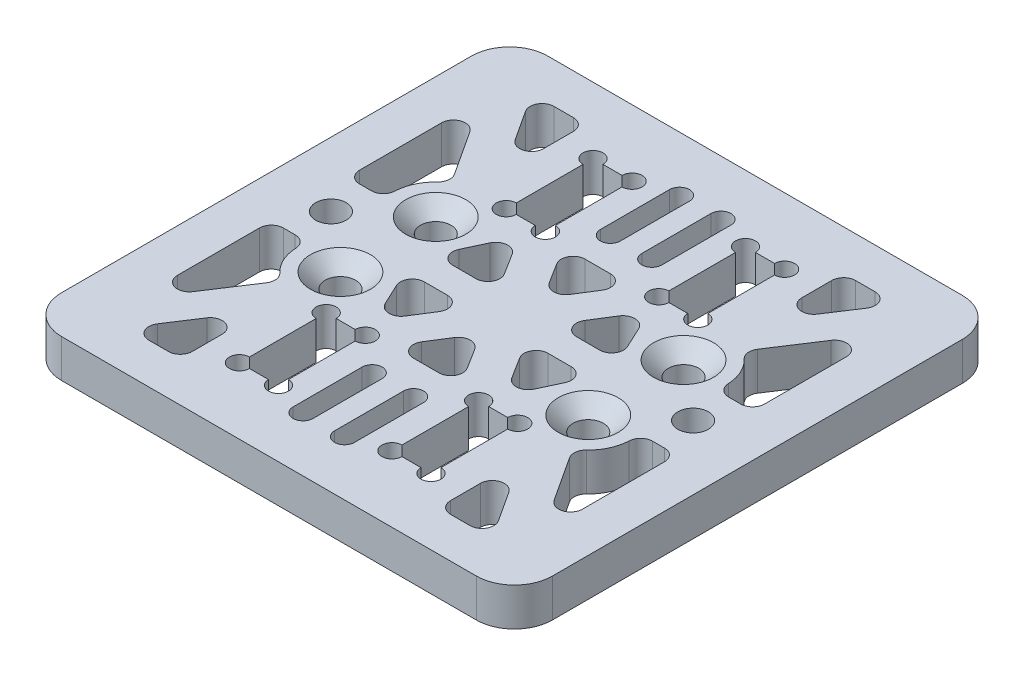
SolidWorks part; units mm, degrees
material "Thornel Mat VMA"
ref_plane "前视基准面" through (0, 0, 0) normal (0, 0, 1) x (1, 0, 0)
ref_plane "上视基准面" through (0, 0, 0) normal (0, 1, 0) x (1, 0, 0)
ref_plane "右视基准面" through (0, 0, 0) normal (1, 0, 0) x (0, 0, -1)
sketch "草图1" plane through (0, 0, 0) normal (0, 1, 0) x (1, 0, 0)
  line L0 (0, 25.5) -> (0, -25.5) construction
  line L1 (-25.75, 25.5) -> (25.75, 25.5)
  line L2 (-25.75, 25.5) -> (-25.75, -25.5)
  line L3 (-25.75, -25.5) -> (25.75, -25.5)
  line L4 (25.75, 25.5) -> (25.75, -25.5)
  line L5 (-25.75, 25.5) -> (25.75, -25.5) construction
  line L6 (-25.75, -25.5) -> (25.75, 25.5) construction
  line L7 (-19, 0) -> (19, 0) construction
  line L8 (-13, 5) -> (-13, -5) construction
  line L9 (22.75, -22.75) -> (-22.75, -22.75) construction
  line L10 (22.75, -22.75) -> (22.75, 22.75) construction
  line L11 (22.75, 22.75) -> (-22.75, 22.75) construction
  line L12 (-22.75, -22.75) -> (-22.75, 22.75) construction
  line L13 (22.75, -22.75) -> (-22.75, 22.75) construction
  line L14 (22.75, 22.75) -> (-22.75, -22.75) construction
  line L15 (13, 5) -> (13, -5) construction
  line L32 (7, 9.45) -> (9, 9.45)
  line L33 (-7, 9.45) -> (-9, 9.45)
  line L34 (-5.95, 10.5) -> (-5.95, 17.5)
  line L35 (-7, 18.55) -> (-9, 18.55)
  line L36 (-10.05, 10.5) -> (-10.05, 17.5)
  line L37 (-5.95, 9.45) -> (-10.05, 18.55) construction
  line L38 (-5.95, 18.55) -> (-10.05, 9.45) construction
  line L39 (5.95, 10.5) -> (5.95, 17.5)
  line L40 (7, 18.55) -> (9, 18.55)
  line L41 (10.05, 10.5) -> (10.05, 17.5)
  line L42 (5.95, 18.55) -> (10.05, 9.45) construction
  line L43 (5.95, 9.45) -> (10.05, 18.55) construction
  line L44 (10.05, -10.5) -> (10.05, -17.5)
  line L45 (7, -18.55) -> (9, -18.55)
  line L46 (5.95, -10.5) -> (5.95, -17.5)
  line L47 (7, -9.45) -> (9, -9.45)
  line L48 (-7, -9.45) -> (-9, -9.45)
  line L49 (-5.95, -10.5) -> (-5.95, -17.5)
  line L50 (-7, -18.55) -> (-9, -18.55)
  line L51 (-10.05, -10.5) -> (-10.05, -17.5)
  circle A0 centre (-19, 0) radius 1.6
  circle A1 centre (19, 0) radius 1.6
  circle A2 centre (-13, 5) radius 1.6
  circle A3 centre (-13, -5) radius 1.6
  circle A4 centre (13, -5) radius 1.6
  circle A5 centre (13, 5) radius 1.6
  arc A14 (-5.95, 17.5) -> (-7, 18.55) centre (-5.95, 18.55) ccw
  arc A15 (-9, 18.55) -> (-10.05, 17.5) centre (-10.05, 18.55) ccw
  arc A16 (-7, 9.45) -> (-5.95, 10.5) centre (-5.95, 9.45) ccw
  arc A17 (-10.05, 10.5) -> (-9, 9.45) centre (-10.05, 9.45) ccw
  arc A18 (10.05, 10.5) -> (9, 9.45) centre (10.05, 9.45) cw
  arc A19 (7, 9.45) -> (5.95, 10.5) centre (5.95, 9.45) cw
  arc A20 (5.95, 17.5) -> (7, 18.55) centre (5.95, 18.55) cw
  arc A21 (9, 18.55) -> (10.05, 17.5) centre (10.05, 18.55) cw
  arc A22 (9, -18.55) -> (10.05, -17.5) centre (10.05, -18.55) ccw
  arc A23 (5.95, -17.5) -> (7, -18.55) centre (5.95, -18.55) ccw
  arc A24 (7, -9.45) -> (5.95, -10.5) centre (5.95, -9.45) ccw
  arc A25 (10.05, -10.5) -> (9, -9.45) centre (10.05, -9.45) ccw
  arc A26 (-10.05, -10.5) -> (-9, -9.45) centre (-10.05, -9.45) cw
  arc A27 (-7, -9.45) -> (-5.95, -10.5) centre (-5.95, -9.45) cw
  arc A28 (-5.95, -17.5) -> (-7, -18.55) centre (-5.95, -18.55) cw
  arc A29 (-9, -18.55) -> (-10.05, -17.5) centre (-10.05, -18.55) cw
  point P0 (0, 0)
  point P13 (0, 0)
  point P31 (-8, 14)
  point P55 (8, 14)
  dimension "D1" = 38
  dimension "D2" = 3.2
  dimension "D4" = 10
  dimension "D5" = 3.2
  dimension "D7" = 3
  dimension "D10" = 2.75
  dimension "D13" = 9
  dimension "D8" = 16
  dimension "D11" = 1.05
  dimension "D3" = 45.5
  dimension "D6" = 9.75
  dimension "D9" = 4.1
  dimension "D12" = 9.1
extrude "凸台-拉伸1" add sketch "草图1" along normal blind 4
sketch "草图4" plane through (0, 4, 0) normal (0, 1, 0) x (1, 0, 0)
  point P0 (-13, 5)
  point P1 (13, 5)
  point P3 (-13, -5)
  point P5 (13, -5)
hole_wizard "M3 锥形沉头孔1" positions "草图4" profile "草图5" countersink size "M3" standard "GB"
sketch "草图5" plane through (-13, 4, -5) normal (1, 0, 0) x (0, 0, 1)
  line L0 (0, 0) -> (0, 4)
  line L1 (0, 4) -> (1.6, 3.0386)
  line L2 (1.6, 3.0386) -> (1.6, 1.55)
  line L3 (1.6, 1.55) -> (3.15, 0)
  line L5 (3.15, 0) -> (0, 0)
  line L6 (-1.6, 1.55) -> (-3.15, 0) construction
  line L10 (0, 4) -> (-1.6, 3.0386) construction
  line L11 (0, -6.35) -> (0, 107.95) construction
  dimension "孔直径" = 3.2
  dimension "孔深度" = 4
  dimension "近端锥形沉头孔直径" = 6.3
  dimension "近端锥形沉头孔角度" = 90
  dimension "导头角度" = 118
sketch "草图7" plane through (0, 4, 0) normal (0, 1, 0) x (1, 0, 0)
  line L0 (22.75, -22.75) -> (-22.75, -22.75) construction
  line L1 (22.75, -22.75) -> (22.75, 22.75) construction
  line L2 (22.75, 22.75) -> (-22.75, 22.75) construction
  line L3 (-22.75, -22.75) -> (-22.75, 22.75) construction
  line L4 (22.75, -22.75) -> (-22.75, -22.75) construction
  line L5 (22.75, -22.75) -> (22.75, 22.75) construction
  line L6 (22.75, 22.75) -> (-22.75, 22.75) construction
  line L7 (-22.75, -22.75) -> (-22.75, 22.75) construction
  line L8 (-5.95, 9.45) -> (5.95, -9.45) construction
  line L9 (-4.4691, 10.3824) -> (7.4309, -8.5176)
  line L10 (-7.4309, 8.5176) -> (4.4691, -10.3824)
  line L11 (-5.95, -9.45) -> (5.95, 9.45) construction
  line L12 (-7.4309, -8.5176) -> (4.4691, 10.3824)
  line L13 (-4.4691, -10.3824) -> (7.4309, 8.5176)
  line L14 (-19, 0) -> (19, 0) construction
  line L19 (0, 25.5) -> (0, -25.5) construction
  line L20 (25.75, 25.5) -> (-25.75, 25.5) construction
  line L21 (-25.75, -25.5) -> (25.75, -25.5) construction
  line L22 (-3.5987, 9) -> (3.5987, 9)
  line L23 (-3.5987, -9) -> (3.5987, -9)
  line L24 (-6.8316, 7.5657) -> (-10.3711, 0)
  line L25 (6.8316, 7.5657) -> (10.3711, 0)
  line L26 (6.8316, -7.5657) -> (10.3711, 0)
  line L27 (-6.8316, -7.5657) -> (-10.3711, 0)
  line L28 (-21.25, 21.25) -> (-21.25, 4)
  line L29 (-21.25, 21.25) -> (-13.55, 21.25)
  line L30 (-21.25, 4) -> (-17.3875, 4)
  line L31 (-13.55, 21.25) -> (-13.55, 9.4663)
  line L32 (-10.05, 17.5) -> (-10.05, 10.5) construction
  line L33 (-21.25, 21.25) -> (-13.55, 9.4663) construction
  line L34 (-19.785, 22.2073) -> (-12.085, 10.4235)
  line L35 (-22.715, 20.2927) -> (-15.015, 8.509)
  line L36 (21.25, 21.25) -> (13.55, 9.4663) construction
  line L37 (19.785, 22.2073) -> (12.085, 10.4235)
  line L38 (22.715, 20.2927) -> (15.015, 8.509)
  line L39 (13.55, 21.25) -> (13.55, 9.4663)
  line L40 (21.25, 21.25) -> (13.55, 21.25)
  line L41 (21.25, 21.25) -> (21.25, 4)
  line L42 (21.25, 4) -> (17.3875, 4)
  line L43 (21.25, -21.25) -> (13.55, -9.4663) construction
  line L44 (19.785, -22.2073) -> (12.085, -10.4235)
  line L45 (22.715, -20.2927) -> (15.015, -8.509)
  line L46 (21.25, -21.25) -> (13.55, -21.25)
  line L47 (21.25, -21.25) -> (21.25, -4)
  line L48 (21.25, -4) -> (17.3875, -4)
  line L49 (13.55, -21.25) -> (13.55, -9.4663)
  line L50 (-21.25, -21.25) -> (-13.55, -9.4663) construction
  line L51 (-19.785, -22.2073) -> (-12.085, -10.4235)
  line L52 (-22.715, -20.2927) -> (-15.015, -8.509)
  line L53 (-13.55, -21.25) -> (-13.55, -9.4663)
  line L54 (-21.25, -21.25) -> (-13.55, -21.25)
  line L55 (-21.25, -21.25) -> (-21.25, -4)
  line L56 (-21.25, -4) -> (-17.3875, -4)
  line L62 (-2.175, 19.75) -> (-2.175, 12.5) construction
  line L63 (-1.125, 19.75) -> (-1.125, 12.5)
  line L68 (-3.225, 19.75) -> (-3.225, 12.5)
  line L69 (2.175, 19.75) -> (2.175, 12.5) construction
  line L72 (1.125, 19.75) -> (1.125, 12.5)
  line L73 (3.225, 19.75) -> (3.225, 12.5)
  line L74 (2.175, -19.75) -> (2.175, -12.5) construction
  line L75 (1.125, -19.75) -> (1.125, -12.5)
  line L76 (3.225, -19.75) -> (3.225, -12.5)
  line L77 (-2.175, -19.75) -> (-2.175, -12.5) construction
  line L78 (-1.125, -19.75) -> (-1.125, -12.5)
  line L79 (-3.225, -19.75) -> (-3.225, -12.5)
  line L80 (-10.3711, 0) -> (10.3711, 0) construction
  line L81 (-10.3711, 1.5) -> (10.3711, 1.5)
  line L82 (-10.3711, -1.5) -> (10.3711, -1.5)
  arc A0 (-4.4691, 10.3824) -> (-7.4309, 8.5176) centre (-5.95, 9.45) ccw
  arc A1 (4.4691, -10.3824) -> (7.4309, -8.5176) centre (5.95, -9.45) ccw
  arc A2 (-7.4309, -8.5176) -> (-4.4691, -10.3824) centre (-5.95, -9.45) ccw
  arc A3 (7.4309, 8.5176) -> (4.4691, 10.3824) centre (5.95, 9.45) ccw
  circle A4 centre (-13, 5) radius 1.6 construction
  arc A5 (-13.55, 9.4663) -> (-17.3875, 4) centre (-13, 5) ccw
  arc A6 (-19.785, 22.2073) -> (-22.715, 20.2927) centre (-21.25, 21.25) ccw
  arc A7 (-15.015, 8.509) -> (-12.085, 10.4235) centre (-13.55, 9.4663) ccw
  arc A8 (19.785, 22.2073) -> (22.715, 20.2927) centre (21.25, 21.25) cw
  arc A9 (15.015, 8.509) -> (12.085, 10.4235) centre (13.55, 9.4663) cw
  arc A10 (13.55, 9.4663) -> (17.3875, 4) centre (13, 5) cw
  arc A11 (19.785, -22.2073) -> (22.715, -20.2927) centre (21.25, -21.25) ccw
  arc A12 (15.015, -8.509) -> (12.085, -10.4235) centre (13.55, -9.4663) ccw
  arc A13 (13.55, -9.4663) -> (17.3875, -4) centre (13, -5) ccw
  arc A14 (-19.785, -22.2073) -> (-22.715, -20.2927) centre (-21.25, -21.25) cw
  arc A15 (-15.015, -8.509) -> (-12.085, -10.4235) centre (-13.55, -9.4663) cw
  arc A16 (-13.55, -9.4663) -> (-17.3875, -4) centre (-13, -5) cw
  arc A17 (-1.125, 19.75) -> (-3.225, 19.75) centre (-2.175, 19.75) ccw
  arc A18 (-3.225, 12.5) -> (-1.125, 12.5) centre (-2.175, 12.5) ccw
  arc A21 (1.125, 19.75) -> (3.225, 19.75) centre (2.175, 19.75) cw
  arc A22 (3.225, 12.5) -> (1.125, 12.5) centre (2.175, 12.5) cw
  arc A23 (1.125, -19.75) -> (3.225, -19.75) centre (2.175, -19.75) ccw
  arc A24 (3.225, -12.5) -> (1.125, -12.5) centre (2.175, -12.5) ccw
  arc A25 (-1.125, -19.75) -> (-3.225, -19.75) centre (-2.175, -19.75) cw
  arc A26 (-3.225, -12.5) -> (-1.125, -12.5) centre (-2.175, -12.5) cw
  arc A27 (-10.3711, 1.5) -> (-10.3711, -1.5) centre (-10.3711, 0) ccw
  arc A28 (10.3711, -1.5) -> (10.3711, 1.5) centre (10.3711, 0) ccw
  point P8 (0, 0)
  point P13 (0, 0)
  point P22 (0, 0)
  point P54 (-17.4, 15.3581)
  point P61 (17.4, 15.3581)
  point P74 (17.4, -15.3581)
  point P87 (-17.4, -15.3581)
  point P98 (-2.175, 16.125)
  point P107 (2.175, 16.125)
  point P112 (0, 0)
  point P115 (2.175, -16.125)
  point P122 (-2.175, -16.125)
  dimension "D3" = 4.5
  dimension "D6" = 3.5
  dimension "D7" = 4.5
  dimension "D10" = 1.05
  dimension "D1" = 3.5
  dimension "D2" = 9
  dimension "D4" = 1.5
  dimension "D5" = 1.5
  dimension "D8" = 3.5
  dimension "D9" = 4
  dimension "D11" = 2.25
  dimension "D12" = 3.5
  dimension "D13" = 3
  dimension "D14" = 3
extrude "切除-拉伸2" cut sketch "草图7" against normal through all contours L29 L34 L31 | A5 L35 L28 L30 | L68 A18 L63 A17 | A22 L73 A21 L72 | L37 L40 L39 | L38 A10 L42 L41 | L22 L9 L12 | L13 L23 L10 | L52 A16 L56 L55 | L51 L54 L53 | A26 L79 A25 L78 | L76 A24 L75 A23 | L49 L46 L44 | A13 L45 L47 L48 | L24 L81 L10 | L13 L81 L25 | L82 L27 L12 | L82 L9 L26
fillet "R1.25 镂空圆角" radius 1.25 46 edges at (3.5987, 2, 9) (-3.5987, 2, 9) (0, 2, 3.2845) (21.25, 2, 4) (21.25, 2, 18.0508) (15.2635, 2, 8.8893) (17.3875, 2, 4) (19.1595, 2, 21.25) (13.55, 2, 21.25) (13.55, 2, 12.6655) (-13.55, 2, 21.25) (-19.1595, 2, 21.25) (-13.55, 2, 12.6655) (-17.3875, 2, 4) (-15.2635, 2, 8.8893) (-21.25, 2, 18.0508) (-21.25, 2, 4) (3.5987, 2, -9) (0, 2, -3.2845) (-3.5987, 2, -9) (21.25, 2, -4) (17.3875, 2, -4) (15.2635, 2, -8.8893) (21.25, 2, -18.0508) (13.55, 2, -12.6655) (19.1595, 2, -21.25) (13.55, 2, -21.25) (-13.55, 2, -21.25) (-13.55, 2, -12.6655) (-19.1595, 2, -21.25) (-17.3875, 2, -4) (-21.25, 2, -4) (-15.2635, 2, -8.8893) (-21.25, 2, -18.0508) (9.6693, 2, 1.5) (6.8316, 2, 7.5657) (3.0124, 2, 1.5) (-3.0124, 2, 1.5) (-6.8316, 2, 7.5657) (-9.6693, 2, 1.5) (9.6693, 2, -1.5) (3.0124, 2, -1.5) (6.8316, 2, -7.5657) (-3.0124, 2, -1.5) (-9.6693, 2, -1.5) (-6.8316, 2, -7.5657)
fillet "R4 外缘圆角" radius 4 4 edges at (-25.75, 2, -25.5) (25.75, 2, -25.5) (-25.75, 2, 25.5) (25.75, 2, 25.5)
